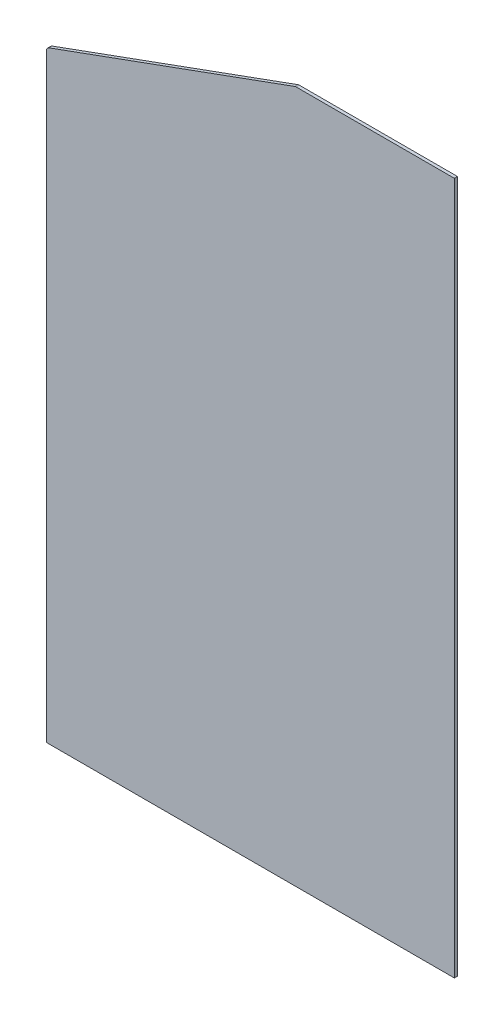
from build123d import *

# Parameters (mm, degrees)
BOSS_EXTRUDE1_DEPTH = 5
FILLET1_R           = 6


with BuildPart() as part:
    # Sketch1 → Boss-Extrude1 (new body)
    with BuildSketch(Plane.XY):
        Polygon((0, 0), (0, 1105.5), (-253.62, 1105.5), (-651, 960.865508307), (-651, 0), align=None)
    extrude(amount=BOSS_EXTRUDE1_DEPTH)

    # Fillet1
    fillet1_edges = [part.edges().sort_by_distance(p)[0] for p in [
        (-651, 960.865508307, 2.5),
        (-253.62, 1105.5, 2.5),
    ]]
    fillet(fillet1_edges, radius=FILLET1_R)


solid = part.part
